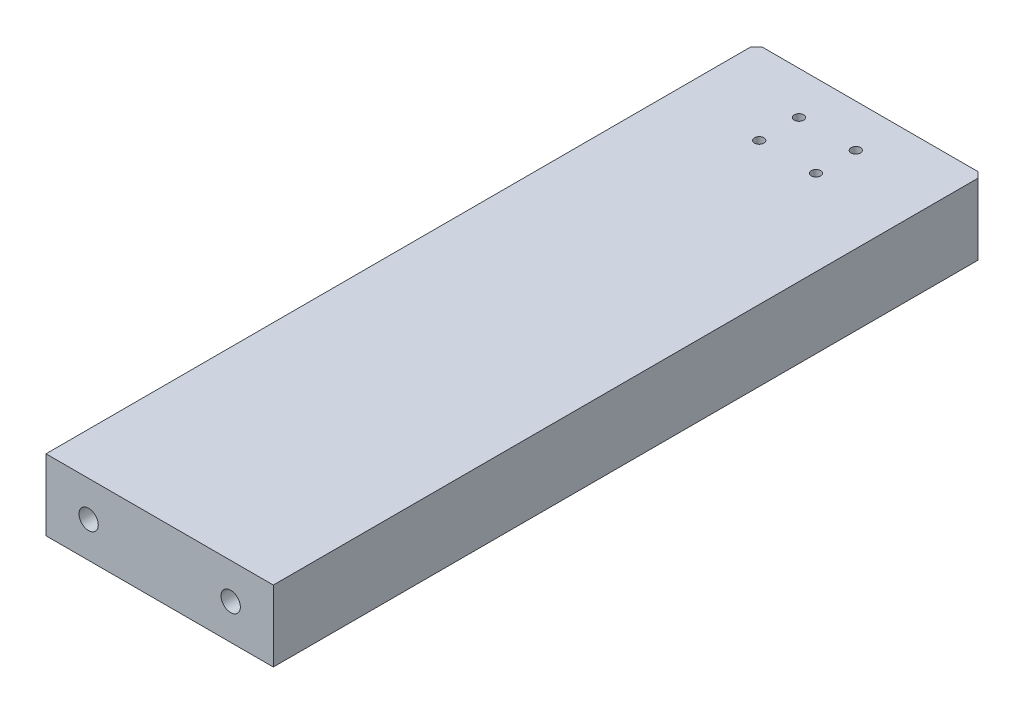
from build123d import *

# Parameters (mm, degrees)
BOSS_EXTRUDE1_DEPTH   = 12.5
CHAMFER1_SIZE         = 2
HOLE1_D               = 9
CUT_EXTRUDE1_DEPTH    = 15
M4_TAPPED_HOLE1_D     = 3.3
SKETCH11_W            = 35
SKETCH11_H            = 25
CUT_EXTRUDE2_DEPTH    = 250.850455273
M8_TAPPED_HOLE2_D     = 6.8
M8_TAPPED_HOLE2_DEPTH = 19.75
M8_TAPPED_HOLE2_TIP   = 2.042926105


with BuildPart() as part:
    # Sketch1 → Boss-Extrude1 (new, symmetric)
    with BuildSketch(Plane(origin=(0, 0, 0), x_dir=(1, 0, 0), z_dir=(0, 1, 0))):
        Polygon((-75, 0), (75, 0), (75, 12), (40, 12), (40, 250), (-40, 250), (-40, 12), (-75, 12), align=None)
    extrude(amount=BOSS_EXTRUDE1_DEPTH, both=True)

    # Chamfer1
    chamfer1_edges = [part.edges().sort_by_distance(p)[0] for p in [
        (-75, 0, -12),
        (-40, 0, -250),
        (40, 0, -250),
        (75, 0, -12),
    ]]
    chamfer(chamfer1_edges, length=CHAMFER1_SIZE)

    # Hole1 (through all)
    with Locations(Plane.XY):
        with Locations((-60, 0), (60, 0)):
            Hole(HOLE1_D / 2)

    # Sketch4 → Cut-Extrude1 (cut)
    with BuildSketch(Plane(origin=(0, -12.5, 0), x_dir=(-1, 0, 0), z_dir=(0, -1, 0))):
        with BuildLine():
            Line((-13.5, 80), (-13.5, 250))
            ThreePointArc((-13.5, 250), (0, 263.5), (13.5, 250))
            Line((13.5, 250), (13.5, 80))
            ThreePointArc((13.5, 80), (0, 66.5), (-13.5, 80))
        make_face()
    extrude(amount=-CUT_EXTRUDE1_DEPTH, mode=Mode.SUBTRACT)

    # M4 Tapped Hole1 (through all)
    with Locations(Plane(origin=(0, 12.5, 0), x_dir=(1, 0, 0), z_dir=(0, 1, 0))):
        with Locations((-10, 235), (-10, 221), (10, 221), (10, 235)):
            Hole(M4_TAPPED_HOLE1_D / 2)

    # Sketch11 → Cut-Extrude2 (cut, through all)
    with BuildSketch(Plane(origin=(0, 0, -12), x_dir=(-1, 0, 0), z_dir=(0, 0, -1))):
        with Locations((-57.5, 0)):
            Rectangle(SKETCH11_W, SKETCH11_H)
        with Locations((57.5, 0)):
            Rectangle(SKETCH11_W, SKETCH11_H)
    extrude(amount=-CUT_EXTRUDE2_DEPTH, mode=Mode.SUBTRACT)

    # M8 Tapped Hole2
    with Locations(Plane.XY):
        with Locations((-25, 0), (25, 0)):
            Hole(M8_TAPPED_HOLE2_D / 2, depth=M8_TAPPED_HOLE2_DEPTH)
            with Locations((0, 0, -(M8_TAPPED_HOLE2_DEPTH + M8_TAPPED_HOLE2_TIP / 2))):  # 118° drill point
                Cone(0, M8_TAPPED_HOLE2_D / 2, M8_TAPPED_HOLE2_TIP, mode=Mode.SUBTRACT)


solid = part.part
